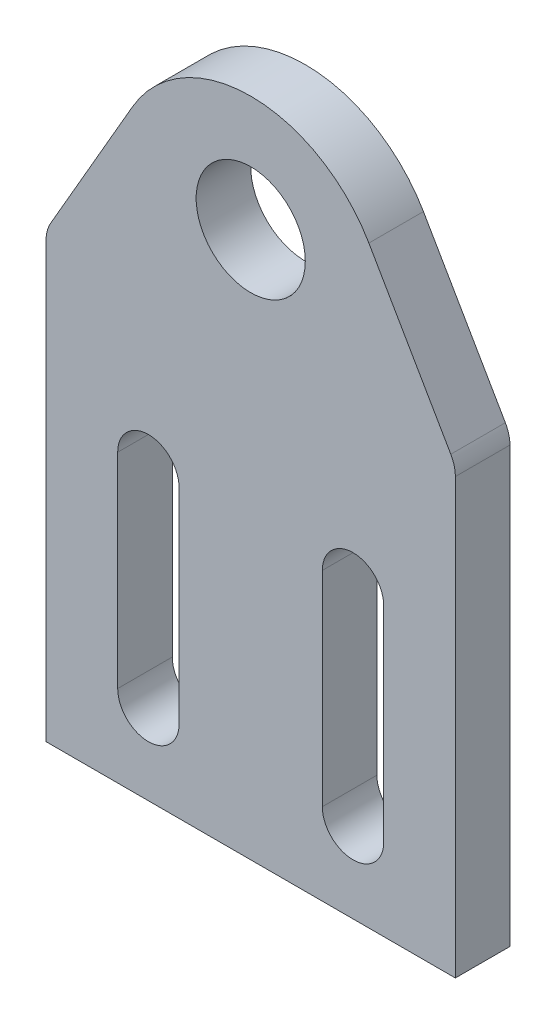
from build123d import *

# Parameters (mm, degrees)
BOSS_EXTRUDE1_DEPTH = 8
SKETCH3_R           = 8
CUT_EXTRUDE1_DEPTH  = 8
CUT_EXTRUDE2_DEPTH  = 115.30458075
FILLET1_R           = 5


with BuildPart() as part:
    # Sketch2 → Boss-Extrude1 (new body)
    with BuildSketch(Plane.XY):
        with BuildLine():
            Line((0, 0), (0, 65))
            Line((0, 65), (12.679491924, 86.961524227))
            ThreePointArc((12.679491924, 86.961524227), (30, 96.961524227), (47.320508076, 86.961524227))
            Line((47.320508076, 86.961524227), (60, 65))
            Line((60, 65), (60, 0))
            Line((60, 0), (0, 0))
        make_face()
    extrude(amount=BOSS_EXTRUDE1_DEPTH)

    # Sketch3 → Cut-Extrude1 (cut)
    with BuildSketch(Plane.XY.offset(8)):
        with Locations((30, 80)):
            Circle(SKETCH3_R)
    extrude(amount=-CUT_EXTRUDE1_DEPTH, mode=Mode.SUBTRACT)

    # Sketch4 → Cut-Extrude2 (cut, through all)
    with BuildSketch(Plane.XY.offset(8)):
        with BuildLine():
            Line((10.5, 12), (10.5, 42))
            ThreePointArc((10.5, 42), (15, 46.5), (19.5, 42))
            Line((19.5, 42), (19.5, 12))
            ThreePointArc((19.5, 12), (15, 7.5), (10.5, 12))
        make_face()
        with BuildLine():
            Line((49.5, 12), (49.5, 42))
            ThreePointArc((49.5, 42), (45, 46.5), (40.5, 42))
            Line((40.5, 42), (40.5, 12))
            ThreePointArc((40.5, 12), (45, 7.5), (49.5, 12))
        make_face()
    extrude(amount=-CUT_EXTRUDE2_DEPTH, mode=Mode.SUBTRACT)

    # Fillet1
    fillet1_edges = [part.edges().sort_by_distance(p)[0] for p in [
        (0, 65, 4),
        (60, 65, 4),
    ]]
    fillet(fillet1_edges, radius=FILLET1_R)


solid = part.part
